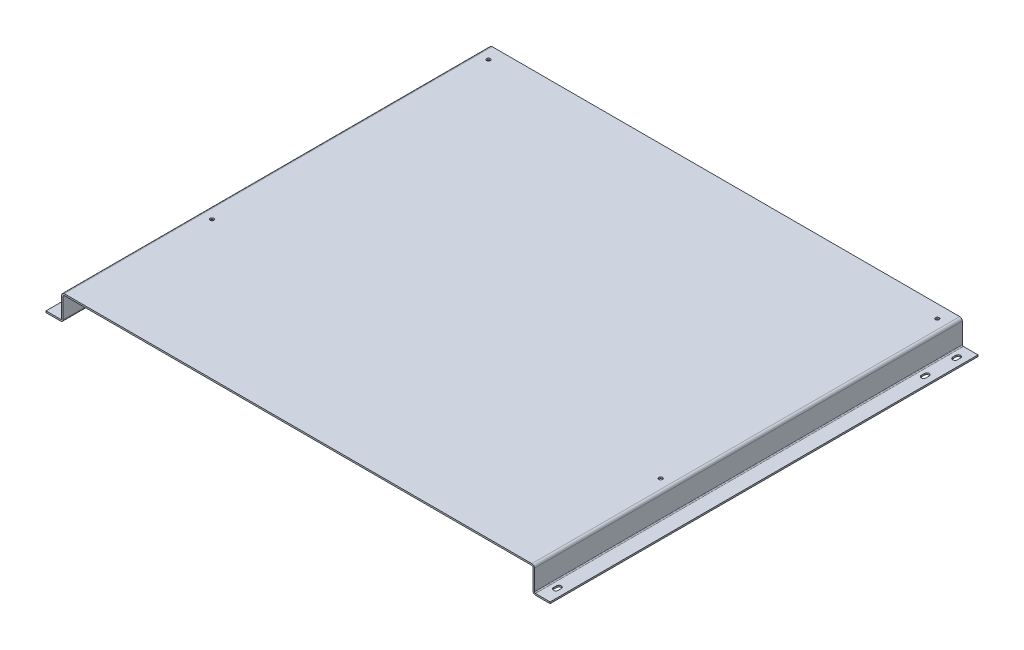
SolidWorks part; units mm, degrees
material "1023 碳钢板 (SS)"
ref_plane "前视基准面" through (0, 0, 0) normal (0, 0, 1) x (1, 0, 0)
ref_plane "上视基准面" through (0, 0, 0) normal (0, 1, 0) x (1, 0, 0)
ref_plane "右视基准面" through (0, 0, 0) normal (1, 0, 0) x (0, 0, -1)
sketch "草图1" plane through (0, 0, 0) normal (0, 0, 1) x (1, 0, 0)
  line L0 (0, 0) -> (28, 0)
  line L1 (30, 2) -> (30, 41)
  line L2 (35, 46) -> (931, 46)
  line L3 (936, 41) -> (936, 2)
  line L4 (938, 0) -> (966, 0)
  line L5 (0, -3) -> (28, -3)
  line L6 (33, 2) -> (33, 41)
  line L7 (35, 43) -> (931, 43)
  line L8 (933, 41) -> (933, 2)
  line L9 (938, -3) -> (966, -3)
  line L10 (0, 0) -> (0, -3)
  line L11 (966, 0) -> (966, -3)
  arc A0 (936, 2) -> (938, 0) centre (938, 2) ccw
  arc A1 (28, 0) -> (30, 2) centre (28, 2) ccw
  arc A2 (30, 41) -> (35, 46) centre (35, 41) cw
  arc A3 (931, 46) -> (936, 41) centre (931, 41) cw
  arc A4 (28, -3) -> (33, 2) centre (28, 2) ccw
  arc A5 (33, 41) -> (35, 43) centre (35, 41) cw
  arc A6 (931, 43) -> (933, 41) centre (931, 41) cw
  arc A7 (933, 2) -> (938, -3) centre (938, 2) ccw
  point P9 (936, 0)
  point P12 (30, 0)
  point P15 (30, 46)
  point P18 (936, 46)
  dimension "D5" = 2
  dimension "D6" = 5
  dimension "D1" = 30
  dimension "D2" = 30
  dimension "D3" = 46
  dimension "D4" = 906
  dimension "D7" = 3
extrude "凸台-拉伸1" add sketch "草图1" along normal blind 820 contours L11 L9 A7 L8 A6 L7 A5 L6 A4 L5 L10 L0 A1 L1 A2 L2 A3 L3 A0 L4
sketch "草图2" plane through (0, 46, 0) normal (0, 1, 0) x (1, 0, 0)
  line L1 (53, -25) -> (913, -25) construction
  line L2 (53, -25) -> (53, -555) construction
  line L3 (53, -555) -> (913, -555) construction
  line L4 (913, -25) -> (913, -555) construction
  line L5 (53, -25) -> (913, -555) construction
  line L6 (53, -555) -> (913, -25) construction
  line L7 (35, 0) -> (931, 0) construction
  circle A0 centre (53, -555) radius 3.5
  circle A1 centre (53, -25) radius 3.5
  circle A2 centre (913, -25) radius 3.5
  circle A3 centre (913, -555) radius 3.5
  point P0 (483, -290)
  point P13 (483, 0)
  dimension "D5" = 7
  dimension "D1" = 860
  dimension "D2" = 530
  dimension "D3" = 25
  dimension "D4" = 25
extrude "切除-拉伸1" cut sketch "草图2" against normal blind 820
sketch "草图3" plane through (0, 0, 0) normal (0, 1, 0) x (1, 0, 0)
  line L7 (0, -820) -> (0, 0) construction
  line L11 (483, 0) -> (483, -481.6892) construction
  line L12 (35, 0) -> (931, 0) construction
  line L22 (0, -410) -> (132.3159, -410) construction
  line L23 (950, -82) -> (950, -88) construction
  line L24 (954.5, -82) -> (954.5, -88)
  line L25 (945.5, -82) -> (945.5, -88)
  line L26 (950, -22) -> (950, -28) construction
  line L27 (954.5, -22) -> (954.5, -28)
  line L28 (945.5, -22) -> (945.5, -28)
  line L29 (16, -82) -> (16, -88) construction
  line L30 (11.5, -82) -> (11.5, -88)
  line L31 (20.5, -82) -> (20.5, -88)
  line L32 (16, -22) -> (16, -28) construction
  line L33 (11.5, -22) -> (11.5, -28)
  line L34 (20.5, -22) -> (20.5, -28)
  line L35 (950, -787) -> (950, -793) construction
  line L36 (954.5, -787) -> (954.5, -793)
  line L37 (945.5, -787) -> (945.5, -793)
  line L38 (16, -787) -> (16, -793) construction
  line L39 (11.5, -787) -> (11.5, -793)
  line L40 (20.5, -787) -> (20.5, -793)
  arc A12 (954.5, -82) -> (945.5, -82) centre (950, -82) ccw
  arc A13 (945.5, -88) -> (954.5, -88) centre (950, -88) ccw
  arc A14 (954.5, -22) -> (945.5, -22) centre (950, -22) ccw
  arc A15 (945.5, -28) -> (954.5, -28) centre (950, -28) ccw
  arc A16 (11.5, -82) -> (20.5, -82) centre (16, -82) cw
  arc A17 (20.5, -88) -> (11.5, -88) centre (16, -88) cw
  arc A18 (11.5, -22) -> (20.5, -22) centre (16, -22) cw
  arc A19 (20.5, -28) -> (11.5, -28) centre (16, -28) cw
  arc A20 (954.5, -787) -> (945.5, -787) centre (950, -787) ccw
  arc A21 (945.5, -793) -> (954.5, -793) centre (950, -793) ccw
  arc A22 (11.5, -787) -> (20.5, -787) centre (16, -787) cw
  arc A23 (20.5, -793) -> (11.5, -793) centre (16, -793) cw
  point P54 (950, -85)
  point P61 (950, -25)
  point P68 (16, -85)
  point P75 (16, -25)
  point P82 (950, -790)
  point P89 (16, -790)
extrude "切除-拉伸2" cut sketch "草图3" against normal blind 10
